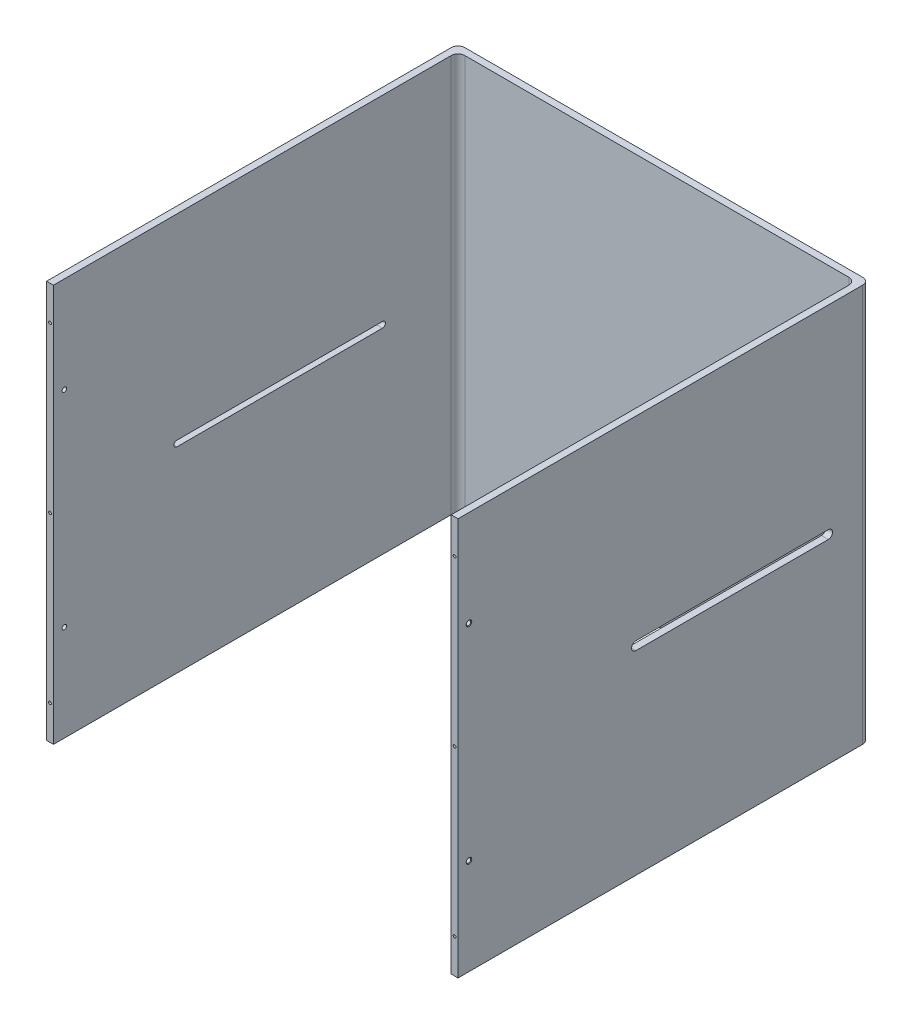
SolidWorks part; units mm, degrees
ref_plane "Front Plane" through (0, 0, 0) normal (0, 0, 1) x (1, 0, 0)
ref_plane "Top Plane" through (0, 0, 0) normal (0, 1, 0) x (1, 0, 0)
ref_plane "Right Plane" through (0, 0, 0) normal (1, 0, 0) x (0, 0, -1)
sketch "Sketch1" plane through (0, 0, 0) normal (0, 1, 0) x (1, 0, 0)
  line L1 (-138.1058, 176.3322) -> (151.8942, 176.3322)
  line L3 (-133.1058, 171.3322) -> (146.8942, 171.3322)
  line L6 (-143.1058, 171.3322) -> (-143.1058, -123.6678)
  line L7 (-143.1058, -123.6678) -> (-138.1058, -123.6678)
  line L8 (-138.1058, 166.3322) -> (-138.1058, -123.6678)
  line L10 (156.8942, 171.3322) -> (156.8942, -123.6678)
  line L11 (156.8942, -123.6678) -> (151.8942, -123.6678)
  line L12 (151.8942, 166.3322) -> (151.8942, -123.6678)
  arc A0 (-133.1058, 171.3322) -> (-138.1058, 166.3322) centre (-133.1058, 166.3322) ccw
  arc A1 (-138.1058, 176.3322) -> (-143.1058, 171.3322) centre (-138.1058, 171.3322) ccw
  arc A2 (151.8942, 176.3322) -> (156.8942, 171.3322) centre (151.8942, 171.3322) cw
  arc A3 (146.8942, 171.3322) -> (151.8942, 166.3322) centre (146.8942, 166.3322) cw
  point P12 (-138.1058, 171.3322)
  point P15 (-143.1058, 176.3322)
  point P18 (156.8942, 176.3322)
  point P21 (151.8942, 171.3322)
  dimension "D7" = 5
  dimension "D8" = 5
  dimension "D1" = 300
  dimension "D2" = 300
  dimension "D3" = 290
  dimension "D4" = 5
  dimension "D5" = 5
  dimension "D6" = 300
extrude "Boss-Extrude1" add sketch "Sketch1" along normal blind 290
hole_wizard "M2.5 Tapped Hole1" positions "Sketch2" profile "Sketch3" tap size "M2.5" standard "GB"
sketch "Sketch2" plane through (0, 0, 123.6678) normal (0, 0, 1) x (1, 0, 0)
  line L0 (-138.1058, 290) -> (-138.1058, 0) construction
  line L2 (-143.1058, 0) -> (-138.1058, 0) construction
  line L3 (156.8942, 290) -> (156.8942, 0) construction
  line L4 (151.8942, 290) -> (156.8942, 290) construction
  point P0 (-140.6058, 145)
  point P2 (-140.6058, 265)
  point P4 (-140.6058, 25)
  point P6 (154.3942, 145)
  point P8 (154.3942, 265)
  point P10 (154.3942, 25)
  dimension "D1" = 2.5
  dimension "D2" = 120
  dimension "D3" = 2.5
  dimension "D4" = 120
  dimension "D5" = 2.5
  dimension "D6" = 145
  dimension "D7" = 2.5
  dimension "D8" = 2.5
  dimension "D9" = 120
  dimension "D10" = 145
  dimension "D11" = 2.5
  dimension "D12" = 120
sketch "Sketch3" plane through (-140.6058, 145, 123.6678) normal (1, 0, 0) x (0, -1, 0)
  line L0 (0, 0) -> (0, 7.8659)
  line L1 (0, 7.8659) -> (1.025, 7.25)
  line L2 (1.025, 7.25) -> (1.025, 0)
  line L5 (1.025, 0) -> (0, 0)
  line L10 (0, 7.8659) -> (-1.025, 7.25) construction
  line L11 (0, -6.35) -> (0, 107.95) construction
  dimension "螺纹孔钻头直径" = 2.05
  dimension "螺纹孔钻头深度" = 7.25
  dimension "导头角度" = 118
cosmetic thread "Hole thread 1" parameters "D1"=5, "D2"=2.5
cosmetic thread "Hole thread 2" parameters "D1"=5, "D2"=2.5
cosmetic thread "Hole thread 3" parameters "D1"=5, "D2"=2.5
cosmetic thread "Hole thread 4" parameters "D1"=5, "D2"=2.5
cosmetic thread "Hole thread 5" parameters "D1"=5, "D2"=2.5
cosmetic thread "Hole thread 6" parameters "D1"=5, "D2"=2.5
sketch "Sketch5" plane through (-143.1058, 0, 0) normal (-1, 0, 0) x (0, 0, 1)
  line L0 (-116.3322, 145) -> (33.6678, 145) construction
  line L1 (-116.3322, 147.1) -> (33.6678, 147.1)
  line L2 (-116.3322, 142.9) -> (33.6678, 142.9)
  line L3 (-171.3322, 290) -> (-171.3322, 0) construction
  line L4 (-171.3322, 290) -> (123.6678, 290) construction
  arc A0 (-116.3322, 147.1) -> (-116.3322, 142.9) centre (-116.3322, 145) ccw
  arc A1 (33.6678, 142.9) -> (33.6678, 147.1) centre (33.6678, 145) ccw
  point P2 (-41.3322, 145)
  dimension "D1" = 2.1
  dimension "D3" = 55
  dimension "D2" = 150
  dimension "D4" = 145
extrude "Cut-Extrude2" cut sketch "Sketch5" against normal blind 41
sketch "Sketch6" plane through (156.8942, 0, 0) normal (1, 0, 0) x (0, 0, -1)
  line L1 (6.0182, 145) -> (146.3322, 145) construction
  line L2 (176.3322, 290) -> (176.3322, 0) construction
  line L3 (6.0182, 148.1) -> (146.3322, 148.1)
  line L4 (6.0182, 141.9) -> (146.3322, 141.9)
  arc A1 (6.0182, 148.1) -> (6.0182, 141.9) centre (6.0182, 145) ccw
  arc A2 (146.3322, 141.9) -> (146.3322, 148.1) centre (146.3322, 145) ccw
  point P7 (76.1752, 145)
  dimension "D1" = 3.1
  dimension "D3" = 30
extrude "Cut-Extrude3" cut sketch "Sketch6" against normal blind 56
hole_wizard "M4 Tapped Hole1" positions "Sketch8" profile "Sketch10" tap size "M4" standard "GB" end condition through all
sketch "Sketch8" plane through (156.8942, 0, 0) normal (1, 0, 0) x (0, 0, -1)
  line L0 (-123.6678, 290) -> (-123.6678, 0) construction
  line L1 (-123.6678, 290) -> (171.3322, 290) construction
  line L2 (-123.6678, 0) -> (171.3322, 0) construction
  point P0 (-115.6678, 220)
  point P2 (-115.6678, 70)
  dimension "D1" = 8
  dimension "D2" = 8
  dimension "D3" = 70
  dimension "D4" = 70
sketch "Sketch10" plane through (156.8942, 220, 115.6678) normal (0, 1, 0) x (0, 0, -1)
  line L0 (0, 0) -> (0, 300)
  line L1 (0, 300) -> (1.65, 300)
  line L2 (1.65, 300) -> (1.65, 0.375)
  line L3 (1.65, 0.375) -> (2.025, 0)
  line L5 (2.025, 0) -> (0, 0)
  line L6 (-1.65, 0.375) -> (-2.025, 0) construction
  line L11 (0, -6.35) -> (0, 107.95) construction
  dimension "通孔螺纹孔钻头直径" = 3.3
  dimension "通孔螺纹孔钻头深度" = 300
  dimension "近端锥形沉头孔直径" = 4.05
  dimension "近端锥形沉头孔角度" = 90
cosmetic thread "Hole thread 7" parameters "D2"=4
cosmetic thread "Hole thread 8" parameters "D2"=4
hole_wizard "M2.5 Tapped Hole2" positions "Sketch11" profile "Sketch12" tap size "M2.5" standard "GB"
sketch "Sketch11" plane through (0, 0, 0) normal (0, -1, 0) x (-1, 0, 0)
  line L0 (-151.8942, 166.3322) -> (-151.8942, -123.6678) construction
  line L1 (-151.8942, -123.6678) -> (-156.8942, -123.6678) construction
  line L3 (133.1058, 171.3322) -> (-146.8942, 171.3322) construction
  line L5 (-6.8942, -828.6678) -> (-6.8942, 49171.3322) construction
  point P0 (-154.3942, 136.3322)
  point P2 (-154.3942, 86.3322)
  point P4 (-154.3942, 6.3322)
  point P6 (-154.3942, -73.6678)
  point P21 (-121.8942, 173.8322)
  point P23 (-51.8942, 173.8322)
  point P44 (-6.8942, 171.3322)
  point P46 (38.1058, 173.8322)
  point P47 (108.1058, 173.8322)
  point P48 (140.6058, -73.6678)
  point P49 (140.6058, 6.3322)
  point P50 (140.6058, 86.3322)
  point P51 (140.6058, 136.3322)
  dimension "D1" = 2.5
  dimension "D2" = 2.5
  dimension "D3" = 2.5
  dimension "D4" = 2.5
  dimension "D5" = 50
  dimension "D6" = 80
  dimension "D7" = 80
  dimension "D8" = 50
  dimension "D9" = 70
  dimension "D10" = 2.5
  dimension "D11" = 2.5
  dimension "D12" = 30
sketch "Sketch12" plane through (154.3942, 0, -136.3322) normal (1, 0, 0) x (0, 0, -1)
  line L0 (0, 0) -> (0, 7.8659)
  line L1 (0, 7.8659) -> (1.025, 7.25)
  line L2 (1.025, 7.25) -> (1.025, 0)
  line L5 (1.025, 0) -> (0, 0)
  line L10 (0, 7.8659) -> (-1.025, 7.25) construction
  line L11 (0, -6.35) -> (0, 107.95) construction
  dimension "螺纹孔钻头直径" = 2.05
  dimension "螺纹孔钻头深度" = 7.25
  dimension "导头角度" = 118
cosmetic thread "Hole thread 9" parameters "D1"=5, "D2"=2.5
cosmetic thread "Hole thread 10" parameters "D1"=5, "D2"=2.5
cosmetic thread "Hole thread 11" parameters "D1"=5, "D2"=2.5
cosmetic thread "Hole thread 12" parameters "D1"=5, "D2"=2.5
cosmetic thread "Hole thread 13" parameters "D1"=5, "D2"=2.5
cosmetic thread "Hole thread 14" parameters "D1"=5, "D2"=2.5
cosmetic thread "Hole thread 15" parameters "D1"=5, "D2"=2.5
cosmetic thread "Hole thread 16" parameters "D1"=5, "D2"=2.5
cosmetic thread "Hole thread 17" parameters "D1"=5, "D2"=2.5
cosmetic thread "Hole thread 18" parameters "D1"=5, "D2"=2.5
cosmetic thread "Hole thread 19" parameters "D1"=5, "D2"=2.5
cosmetic thread "Hole thread 20" parameters "D1"=5, "D2"=2.5
